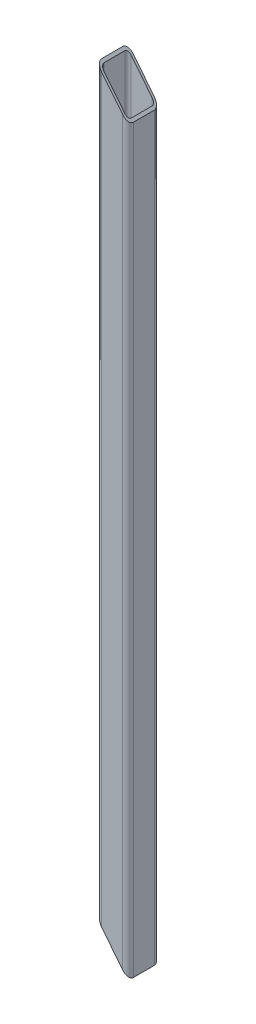
from build123d import *

# Parameters (mm, degrees)
BOSS_EXTRUDE1_DEPTH     = 2000
CUT_EXTRUDE1_DEPTH      = 2002.124683772
CUT_EXTRUDE1_DEPTH_BACK = 2002.124683772


with BuildPart() as part:
    # Sketch1 → Boss-Extrude1 (new body)
    with BuildSketch(Plane(origin=(0, 0, 0), x_dir=(1, 0, 0), z_dir=(0, 1, 0))):
        with BuildLine():
            Line((-20, -30), (20, -30))
            ThreePointArc((20, -30), (27.071067812, -27.071067812), (30, -20))
            Line((30, -20), (30, 20))
            ThreePointArc((30, 20), (27.071067812, 27.071067812), (20, 30))
            Line((20, 30), (-20, 30))
            ThreePointArc((-20, 30), (-27.071067812, 27.071067812), (-30, 20))
            Line((-30, 20), (-30, -20))
            ThreePointArc((-30, -20), (-27.071067812, -27.071067812), (-20, -30))
        make_face()
        with BuildLine():
            Line((-26, -20), (-26, 20))
            ThreePointArc((-26, 20), (-24.242640687, 24.242640687), (-20, 26))
            Line((-20, 26), (20, 26))
            ThreePointArc((20, 26), (24.242640687, 24.242640687), (26, 20))
            Line((26, 20), (26, -20))
            ThreePointArc((26, -20), (24.242640687, -24.242640687), (20, -26))
            Line((20, -26), (-20, -26))
            ThreePointArc((-20, -26), (-24.242640687, -24.242640687), (-26, -20))
        make_face(mode=Mode.SUBTRACT)
    extrude(amount=BOSS_EXTRUDE1_DEPTH)

    # Sketch2 → Cut-Extrude1 (cut, two sides: drawn at the far end of the back side and taken through both)
    with BuildSketch(Plane.XY.offset(30).offset(-CUT_EXTRUDE1_DEPTH_BACK)):
        Polygon((30, 0), (-30, 75.027298751), (-170.24369385, -210.007574385), align=None)
        Polygon((-30, 1484.027298751), (30, 1409), (525.992052796, 1638.556238223), (8.977575366, 2080.626411119), (-421.015295507, 1818.362615914), align=None)
    extrude(amount=CUT_EXTRUDE1_DEPTH + CUT_EXTRUDE1_DEPTH_BACK, mode=Mode.SUBTRACT)


solid = part.part
